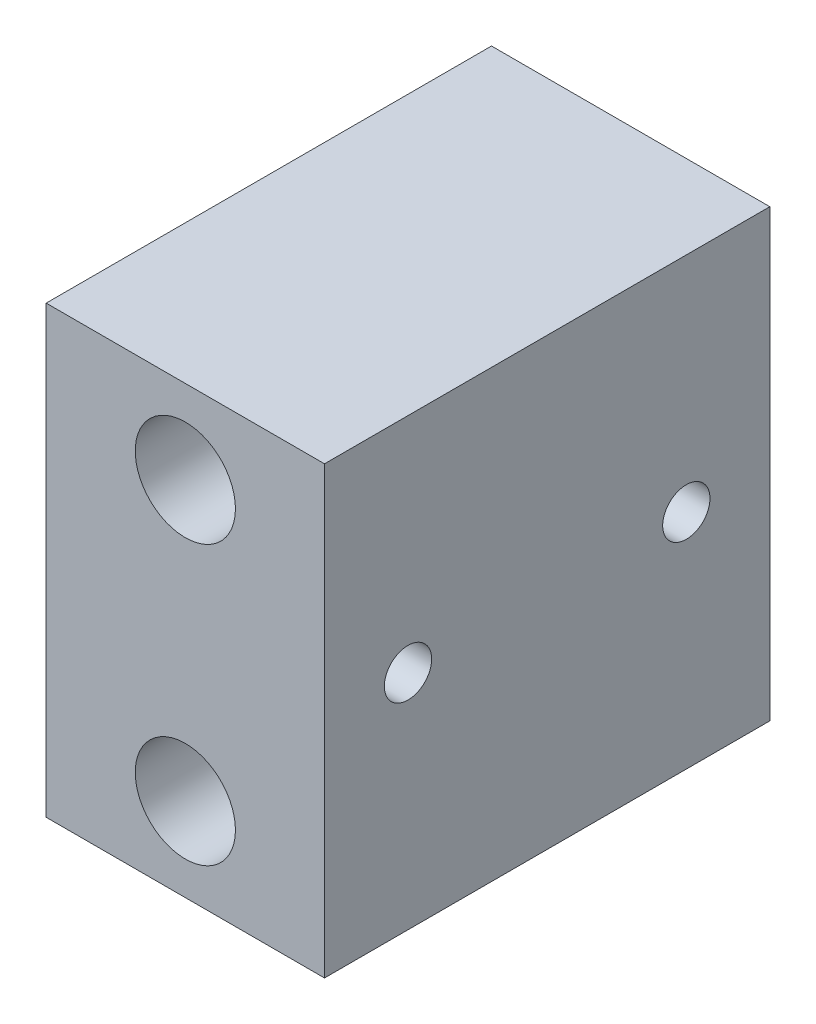
SolidWorks part; units mm, degrees
ref_plane "前视基准面" through (0, 0, 0) normal (0, 0, 1) x (1, 0, 0)
ref_plane "上视基准面" through (0, 0, 0) normal (0, 1, 0) x (1, 0, 0)
ref_plane "右视基准面" through (0, 0, 0) normal (1, 0, 0) x (0, 0, -1)
sketch "草图1" plane through (0, 0, 0) normal (1, 0, 0) x (0, 0, -1)
  line L1 (-40, 40) -> (40, 40)
  line L2 (-40, 40) -> (-40, -40)
  line L3 (-40, -40) -> (40, -40)
  line L4 (40, 40) -> (40, -40)
  line L5 (-40, 40) -> (40, -40) construction
  line L6 (-40, -40) -> (40, 40) construction
  point P0 (0, 0)
  dimension "D1" = 80
  dimension "D2" = 80
extrude "凸台-拉伸1" add sketch "草图1" along normal blind 50
hole_wizard "打孔尺寸(%根据)内六角圆柱头螺钉的类型1" positions "草图2" profile "草图3" counterbore size "M10" standard "GB" end condition through all
sketch "草图2" plane through (0, 0, 40) normal (0, 0, 1) x (1, 0, 0)
  line L0 (25, 40) -> (25, -42.848) construction
  line L1 (50, 40) -> (0, 40) construction
  line L3 (0, 0) -> (80.871, 0) construction
  point P0 (25, 25)
  point P2 (25, -25)
  dimension "D1" = 50
sketch "草图3" plane through (25, 25, 40) normal (1, 0, 0) x (0, -1, 0)
  line L0 (0, 0) -> (0, 80)
  line L1 (0, 80) -> (5.5, 80)
  line L3 (5.5, 80) -> (5.5, 30)
  line L4 (5.5, 30) -> (9, 30)
  line L5 (9, 30) -> (9, 0)
  line L7 (9, 0) -> (0, 0)
  line L11 (0, -6.35) -> (0, 107.95) construction
  dimension "通孔孔直径" = 11
  dimension "通孔孔深度" = 80
  dimension "柱形沉头孔直径" = 18
  dimension "柱形沉头孔深度" = 30
hole_wizard "M10 螺纹孔1" positions "草图4" profile "草图5" tap size "M10" standard "GB" end condition through all
sketch "草图4" plane through (50, 0, 0) normal (1, 0, 0) x (0, 0, -1)
  line L0 (0, -40) -> (0, 48.9377) construction
  line L1 (-40, -40) -> (40, -40) construction
  point P0 (25, 0)
  point P6 (-25, 0)
  dimension "D1" = 50
sketch "草图5" plane through (50, 0, -25) normal (0, 1, 0) x (0, 0, -1)
  line L0 (0, 0) -> (0, 50)
  line L1 (0, 50) -> (4.25, 50)
  line L2 (4.25, 50) -> (4.25, 0)
  line L5 (4.25, 0) -> (0, 0)
  line L11 (0, -6.35) -> (0, 107.95) construction
  dimension "通孔螺纹孔钻头直径" = 8.5
  dimension "通孔螺纹孔钻头深度" = 50
cosmetic thread "孔螺蚊线1" parameters "D2"=10
cosmetic thread "孔螺蚊线2" parameters "D2"=10
